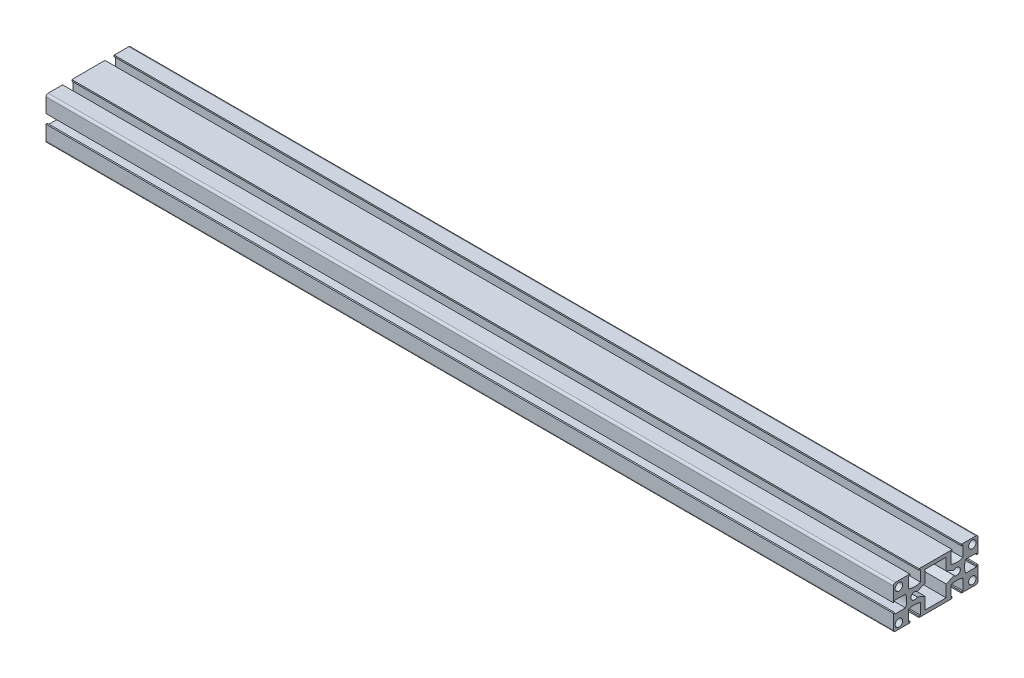
SolidWorks part; units mm, degrees
ref_plane "前视基准面" through (0, 0, 0) normal (0, 0, 1) x (1, 0, 0)
ref_plane "上视基准面" through (0, 0, 0) normal (0, 1, 0) x (1, 0, 0)
ref_plane "右视基准面" through (0, 0, 0) normal (1, 0, 0) x (0, 0, -1)
sketch "草图1" plane through (0, 0, 0) normal (0, 0, 1) x (1, 0, 0)
  line L0 (-300, 0) -> (300, 0)
  point P4 (0, 0)
  dimension "D1" = 600
other "工业铝型材 30 X 60G X R1.5(1)"
ref_plane "基准面1" through (-300, 0, 0) normal (1, 0, 0) x (0, 1, 0)
sketch "Sketch1" plane through (-300, 0, 0) normal (1, 0, 0) x (0, 1, 0)
  line L0 (-3.25, 30) -> (-3.25, 29)
  line L1 (-13.5, 30) -> (-3.25, 30)
  line L2 (-15, 28.5) -> (-15, 18.25)
  line L3 (-13.5, -30) -> (-3.25, -30)
  line L4 (15, 28.5) -> (15, 18.25)
  line L5 (-12.5, 7.5) -> (-4, 7.5)
  line L6 (-12.5, 7.5) -> (-12.5, -7.5)
  line L7 (-12.5, -7.5) -> (-4, -7.5)
  line L8 (0, 30) -> (0, 0) construction
  line L9 (0, 0) -> (15, 0) construction
  line L10 (12.5, 7.5) -> (12.5, -7.5)
  line L11 (-3.25, 29) -> (-4.25, 29)
  line L12 (-4.25, 29) -> (-4.25, 21.2778)
  line L13 (-11, 26) -> (-15, 30) construction
  line L14 (4.25, 29) -> (4.25, 21.2778)
  line L15 (3.25, 29) -> (4.25, 29)
  line L16 (3.25, 30) -> (3.25, 29)
  line L17 (3.25, 30) -> (13.5, 30)
  line L18 (-1.6656, 13.1357) -> (-4, 7.5)
  line L19 (1.6656, 13.1357) -> (4, 7.5)
  line L20 (4, 7.5) -> (12.5, 7.5)
  line L21 (1.6656, -13.1357) -> (4, -7.5)
  line L22 (-1.6656, -13.1357) -> (-4, -7.5)
  line L23 (4, -7.5) -> (12.5, -7.5)
  line L24 (15, 18.25) -> (14, 18.25)
  line L25 (14, 18.25) -> (14, 19.25)
  line L26 (14, 19.25) -> (6.2778, 19.25)
  line L27 (14, 10.75) -> (6.2778, 10.75)
  line L28 (14, 11.75) -> (14, 10.75)
  line L29 (15, 11.75) -> (14, 11.75)
  line L30 (3.25, 0) -> (3.25, 1) [skipped]
  line L31 (3.25, 1) -> (4.25, 1) [skipped]
  line L32 (4.25, 1) -> (4.25, 8.7222) [skipped]
  line L33 (-4.25, 1) -> (-4.25, 8.7222) [skipped]
  line L34 (-3.25, 1) -> (-4.25, 1) [skipped]
  line L35 (-3.25, 0) -> (-3.25, 1) [skipped]
  line L36 (-15, 11.75) -> (-14, 11.75)
  line L37 (-14, 11.75) -> (-14, 10.75)
  line L38 (-14, 10.75) -> (-6.2778, 10.75)
  line L39 (-14, 19.25) -> (-6.2778, 19.25)
  line L40 (-14, 18.25) -> (-14, 19.25)
  line L41 (-15, 18.25) -> (-14, 18.25)
  line L42 (-15, 11.75) -> (-15, -11.75)
  line L43 (15, 11.75) -> (15, -11.75)
  line L44 (-15, -18.25) -> (-14, -18.25)
  line L45 (-14, -18.25) -> (-14, -19.25)
  line L46 (-14, -19.25) -> (-6.2778, -19.25)
  line L47 (-14, -10.75) -> (-6.2778, -10.75)
  line L48 (-14, -11.75) -> (-14, -10.75)
  line L49 (-15, -11.75) -> (-14, -11.75)
  line L50 (15, -11.75) -> (14, -11.75)
  line L51 (14, -11.75) -> (14, -10.75)
  line L52 (14, -10.75) -> (6.2778, -10.75)
  line L53 (14, -19.25) -> (6.2778, -19.25)
  line L54 (14, -18.25) -> (14, -19.25)
  line L55 (15, -18.25) -> (14, -18.25)
  line L56 (3.25, -30) -> (3.25, -29)
  line L57 (3.25, -29) -> (4.25, -29)
  line L58 (4.25, -29) -> (4.25, -21.2778)
  line L59 (-4.25, -29) -> (-4.25, -21.2778)
  line L60 (-3.25, -29) -> (-4.25, -29)
  line L61 (-3.25, -30) -> (-3.25, -29)
  line L62 (3.25, -30) -> (13.5, -30)
  line L63 (-15, -18.25) -> (-15, -28.5)
  line L64 (15, -18.25) -> (15, -28.5)
  arc A0 (-4.25, 21.2778) -> (4.25, 21.2778) centre (0, 32.5) ccw
  circle A1 centre (-11, 26) radius 2.65
  circle A2 centre (11, 26) radius 2.65
  arc A3 (-15, 28.5) -> (-13.5, 30) centre (-13.5, 28.5) cw
  arc A4 (15, 28.5) -> (13.5, 30) centre (13.5, 28.5) ccw
  arc A5 (15, -28.5) -> (13.5, -30) centre (13.5, -28.5) cw
  arc A6 (-13.5, -30) -> (-15, -28.5) centre (-13.5, -28.5) cw
  arc A7 (1.6656, 13.1357) -> (-1.6656, 13.1357) centre (0, 15) ccw
  arc A8 (-1.6656, -13.1357) -> (1.6656, -13.1357) centre (0, -15) ccw
  arc A9 (6.2778, 19.25) -> (6.2778, 10.75) centre (17.5, 15) ccw
  arc A10 (4.25, 8.7222) -> (-4.25, 8.7222) centre (0, -2.5) ccw [skipped]
  arc A11 (-6.2778, 10.75) -> (-6.2778, 19.25) centre (-17.5, 15) ccw
  arc A12 (-6.2778, -10.75) -> (-6.2778, -19.25) centre (-17.5, -15) cw
  arc A13 (6.2778, -19.25) -> (6.2778, -10.75) centre (17.5, -15) cw
  circle A14 centre (11, -26) radius 2.65
  arc A15 (-4.25, -21.2778) -> (4.25, -21.2778) centre (0, -32.5) cw
  circle A16 centre (-11, -26) radius 2.65
  point P102 (15, -30)
  point P103 (-15, -30)
  point P104 (0, 0)
  dimension "D1" = 60
  dimension "D2" = 30
  dimension "D3" = 15
  dimension "D4" = 2.5
  dimension "D5" = 6.5
  dimension "D6" = 8.5
  dimension "D7" = 12
  dimension "D8" = 1
  dimension "D10" = 5.3
  dimension "D11" = 4
  dimension "D12" = 1.5
  dimension "D13" = 5
  dimension "D14" = 30
  dimension "D9" = 9.5
  dimension "D15" = 45
  dimension "D16" = 8
